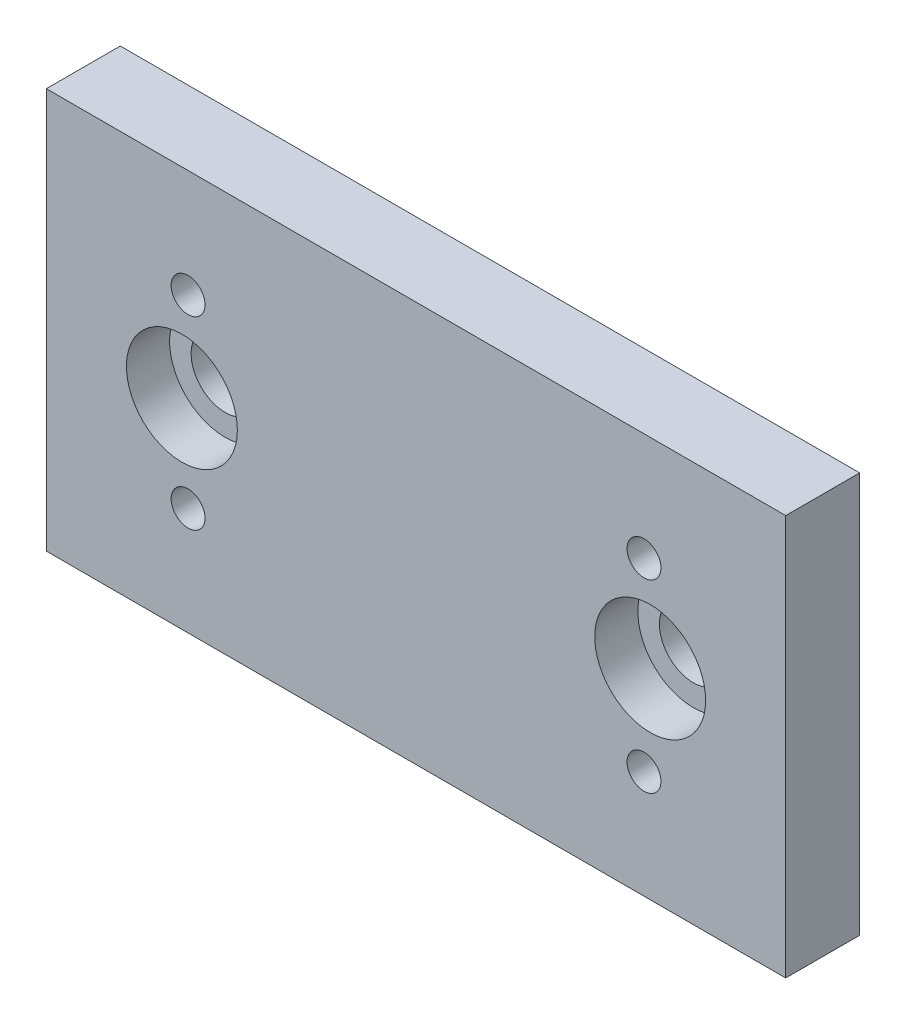
SolidWorks part; units mm, degrees
ref_plane "Front Plane" through (0, 0, 0) normal (0, 0, 1) x (1, 0, 0)
ref_plane "Top Plane" through (0, 0, 0) normal (0, 1, 0) x (1, 0, 0)
ref_plane "Right Plane" through (0, 0, 0) normal (1, 0, 0) x (0, 0, -1)
sketch "Sketch1" plane through (0, 0, 0) normal (0, 0, 1) x (1, 0, 0)
  line L1 (-60, 32.5) -> (60, 32.5)
  line L2 (-60, 32.5) -> (-60, -32.5)
  line L3 (-60, -32.5) -> (60, -32.5)
  line L4 (60, 32.5) -> (60, -32.5)
  line L5 (-60, 32.5) -> (60, -32.5) construction
  line L6 (-60, -32.5) -> (60, 32.5) construction
  point P0 (0, 0)
  dimension "D1" = 120
  dimension "D2" = 65
extrude "Boss-Extrude1" add sketch "Sketch1" along normal blind 12
hole_wizard "Hole for Torx socket cap screw1" positions "Sketch3" profile "Sketch2" counterbore size "M10" standard "GB" end condition through all
sketch "Sketch3" plane through (0, 0, 12) normal (0, 0, 1) x (1, 0, 0)
  point P1 (-38, 0)
  point P5 (38, 0)
  dimension "D1" = 38
  dimension "D2" = 38
sketch "Sketch2" plane through (-38, 0, 12) normal (1, 0, 0) x (0, -1, 0)
  line L0 (0, 0) -> (0, 12)
  line L1 (0, 12) -> (5.5, 12)
  line L3 (5.5, 12) -> (5.5, 7)
  line L4 (5.5, 7) -> (9, 7)
  line L5 (9, 7) -> (9, 0)
  line L7 (9, 0) -> (0, 0)
  line L11 (0, -6.35) -> (0, 107.95) construction
  dimension "通孔孔直径" = 11
  dimension "通孔孔深度" = 12
  dimension "柱形沉头孔直径" = 18
  dimension "柱形沉头孔深度" = 7
hole_wizard "Hole for socket head cap screw, type2" positions "Sketch5" profile "Sketch4" counterbore size "M5" standard "GB"
sketch "Sketch5" plane through (0, 0, 0) normal (0, 0, -1) x (-1, 0, 0)
  point P1 (-37, 15)
  point P5 (-37, -15)
  point P9 (37, -15)
  point P13 (37, 15)
  dimension "D1" = 37
  dimension "D2" = 37
  dimension "D3" = 15
  dimension "D4" = 15
sketch "Sketch4" plane through (37, 15, 0) normal (1, 0, 0) x (0, 1, 0)
  line L0 (0, 0) -> (0, 12)
  line L1 (0, 12) -> (2.75, 12)
  line L3 (2.75, 12) -> (2.75, 5.7)
  line L4 (2.75, 5.7) -> (5, 5.7)
  line L5 (5, 5.7) -> (5, 0)
  line L7 (5, 0) -> (0, 0)
  line L11 (0, -6.35) -> (0, 107.95) construction
  dimension "通孔孔直径" = 5.5
  dimension "通孔孔深度" = 12
  dimension "柱形沉头孔直径" = 10
  dimension "柱形沉头孔深度" = 5.7
